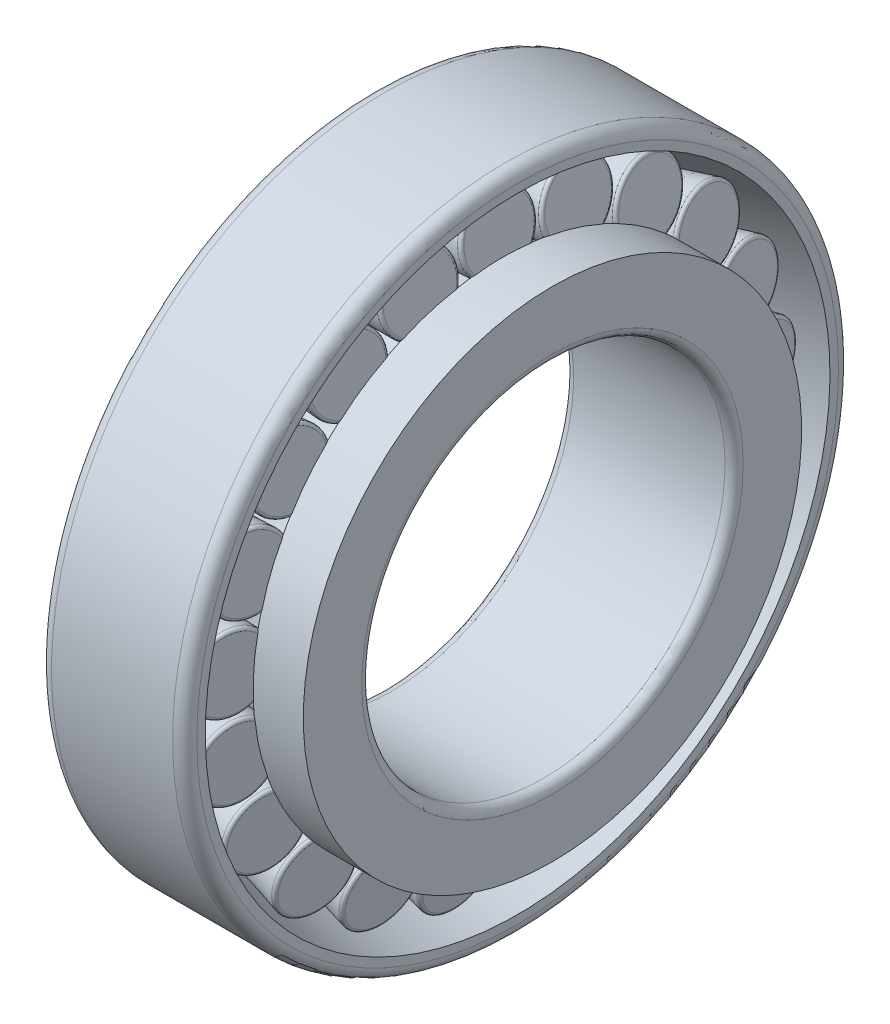
SolidWorks part; units mm, degrees
ref_plane "Front" through (0, 0, 0) normal (0, 0, 1) x (1, 0, 0)
ref_plane "Top" through (0, 0, 0) normal (0, 1, 0) x (1, 0, 0)
ref_plane "Right" through (0, 0, 0) normal (1, 0, 0) x (0, 0, -1)
other "Configuration Table"
sketch "Sketch1" plane through (0, 0, 0) normal (0, 0, 1) x (1, 0, 0)
  line L0 (17.75, 0) -> (13.9916, 0) construction
  line L1 (12, 51.5977) -> (12, 53)
  line L2 (10, 55) -> (-10, 55)
  line L3 (-12, 53) -> (-12, 45.118)
  line L4 (-12, 45.118) -> (12, 51.5977)
  line L5 (-10.25, 31.5) -> (-10.25, 38.1312)
  line L6 (-8.75, 30) -> (16.25, 30)
  line L7 (17.75, 31.5) -> (17.75, 41.1595)
  line L8 (-7.0936, 36.6312) -> (-8.7625, 45.9921)
  line L9 (10, 38.1595) -> (7.806, 50.4654)
  line L10 (-7.928, 41.3116) -> (8.903, 44.3124) construction
  line L11 (-7.0936, 36.6312) -> (10, 38.1595)
  line L12 (9.4651, 42.5) -> (17.75, 42.5)
  line L13 (17.75, 41.1595) -> (9.4651, 41.1595)
  line L14 (-10.25, 38.1312) -> (-7.361, 38.1312)
  arc A0 (-10, 55) -> (-12, 53) centre (-10, 53) ccw
  arc A1 (12, 53) -> (10, 55) centre (10, 53) ccw
  arc A2 (-8.75, 30) -> (-10.25, 31.5) centre (-8.75, 31.5) cw
  arc A3 (16.25, 30) -> (17.75, 31.5) centre (16.25, 31.5) ccw
  point P19 (-12, 55)
  point P22 (12, 55)
  point P24 (0, 55)
  point P29 (-10.25, 30)
  point P32 (17.75, 30)
revolve "Revolve1" add sketch "Sketch1" angle 360 about L0
sketch "Sketch2" plane through (0, 0, 0) normal (0, 0, 1) x (1, 0, 0)
  line L0 (-7.9477, 41.3081) -> (5.8893, 43.7751) construction
  line L4 (-7.928, 41.3116) -> (8.903, 44.3124) construction
  line L5 (-7.9477, 41.3081) -> (8.9227, 44.3159)
  line L7 (-8.7822, 45.9886) -> (-7.11, 36.6096)
  line L8 (10.0235, 38.1415) -> (7.8257, 50.4689)
  line L9 (-7.11, 36.6096) -> (10.0235, 38.1415)
  line L10 (-7.9477, 41.3081) -> (-7.1904, 37.0607)
  line L11 (9.9277, 38.6787) -> (8.9227, 44.3159)
  line L12 (-6.6537, 36.6504) -> (9.48, 38.0929)
  arc A0 (-6.6537, 36.6504) -> (-7.1904, 37.0607) centre (-6.6982, 37.1485) cw
  arc A1 (9.48, 38.0929) -> (9.9277, 38.6787) centre (9.4355, 38.5909) ccw
revolve "Revolve2" add sketch "Sketch2" angle 360 about L0
sketch "Sketch3" plane through (0, 0, 0) normal (0, 0, 1) x (1, 0, 0)
  line L0 (-12, 45.118) -> (12, 51.5977) construction
  line L1 (-12, 53) -> (-12, 45.118) construction
  line L2 (10, 55) -> (-10, 55) construction
  line L3 (12, 51.5977) -> (12, 53) construction
  line L4 (-12, 45.118) -> (12, 51.5977)
  line L5 (-12, 53) -> (-12, 45.118)
  line L6 (10, 55) -> (-10, 55)
  line L7 (12, 51.5977) -> (12, 53)
  arc A0 (-10, 55) -> (-12, 53) centre (-10, 53) ccw construction
  arc A1 (12, 53) -> (10, 55) centre (10, 53) ccw construction
  arc A2 (-10, 55) -> (-12, 53) centre (-10, 53) ccw
  arc A3 (12, 53) -> (10, 55) centre (10, 53) ccw
revolve "Revolve3" add sketch "Sketch3" angle 360 about axis through (17.75, 0, 0) along (-1, 0, 0)
pattern_circular "Circular-Pattern1" count 21 over 360 about axis through (0, 0, 0) along (1, 0, 0) of "Revolve2"
equation "\"gzzj@Sketch1\" =  ( \"DD@Sketch1\" - \"XD@Sketch1\" )  / 4"
equation "\"D1@Sketch1\" = \"DB@Sketch1\" - \"DT@Sketch1\" / 20"
equation "\"D2@Sketch1\" = \"DT@Sketch1\" - \"DC@Sketch1\" + \"XR12@Sketch1\""
equation "\"D4@Sketch1\" = \"D3@Sketch1\" / 2"
equation "\"D2@Sketch2\" = \"gzzj@Sketch1\" / 25"
equation "\"ZJ@Sketch1\" =  ( \"DD@Sketch1\" + \"XD@Sketch1\" )  / 2"
equation "\"D1@Circular-Pattern1\" = int( 3.14159265 / atn(( \"gzzj@Sketch1\" / 2) / sqr( \"ZJ@Sketch1\" * \"ZJ@Sketch1\" /4 - ( \"gzzj@Sketch1\"/ 2) *  ( \"gzzj@Sketch1\"/ 2))))"
